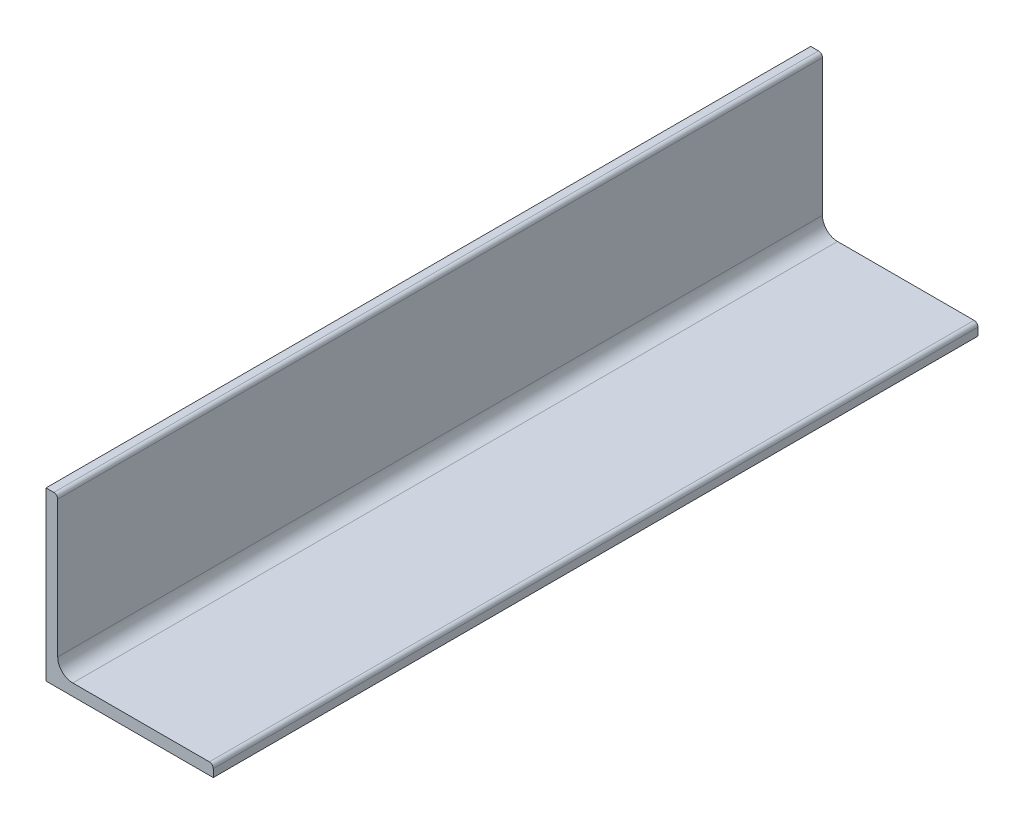
from build123d import *

# Parameters (mm, degrees)
BOSS_EXTRUDE1_DEPTH = 457.2


with BuildPart() as part:
    # Sketch1 → Boss-Extrude1 (new, symmetric)
    with BuildSketch(Plane.XY):
        with BuildLine():
            Line((0, 200), (0, 0))
            Line((0, 0), (200, 0))
            Line((200, 0), (200, 9.333333333))
            ThreePointArc((200, 9.333333333), (198.633164979, 12.633164979), (195.333333333, 14))
            Line((195.333333333, 14), (32, 14))
            ThreePointArc((32, 14), (19.272077939, 19.272077939), (14, 32))
            Line((14, 32), (14, 195.333333333))
            ThreePointArc((14, 195.333333333), (12.633164979, 198.633164979), (9.333333333, 200))
            Line((9.333333333, 200), (0, 200))
        make_face()
    extrude(amount=BOSS_EXTRUDE1_DEPTH, both=True)


solid = part.part
